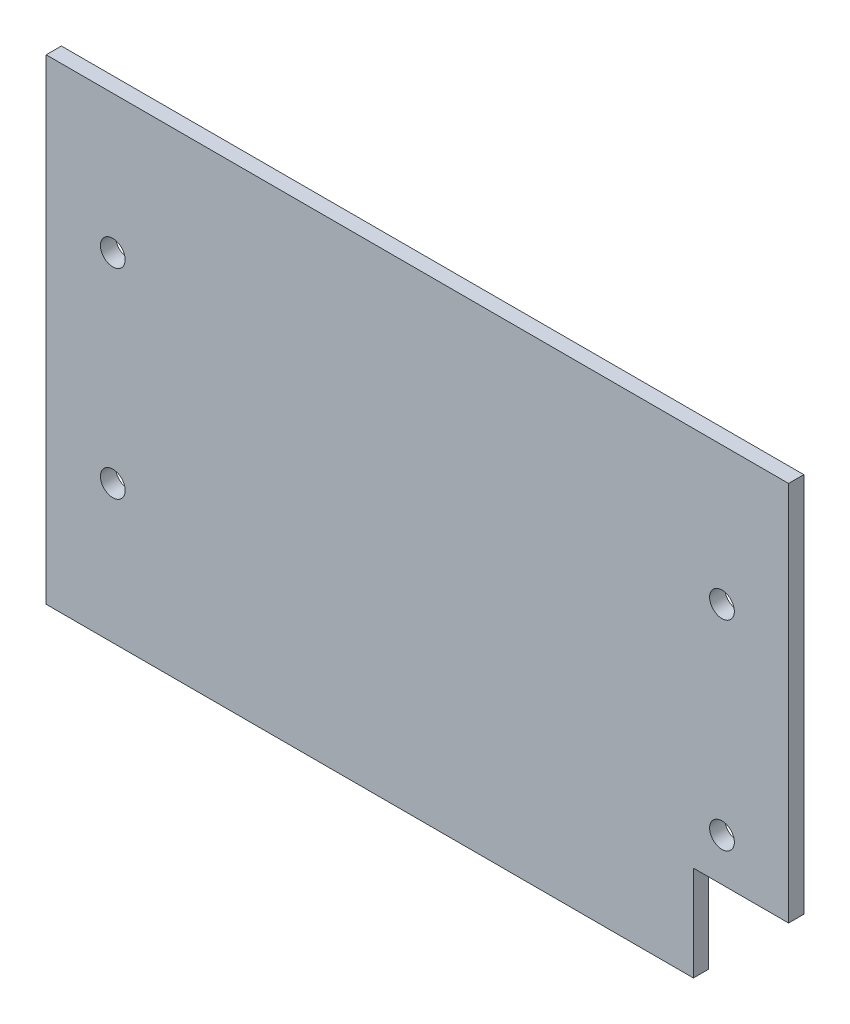
from build123d import *

# Parameters (mm, degrees)
SKETCH_1_W          = 390
SKETCH_1_H          = 250
EXTRUDE_1_DEPTH     = 8
CUT_EXTRUDE_1_DEPTH = 8
SKETCH_3_W          = 50
SKETCH_3_H          = 50
CUT_EXTRUDE_2_DEPTH = 60


with BuildPart() as part:
    # 草图1 → 凸台-拉伸1 (new body)
    with BuildSketch(Plane.XY):
        with Locations((195, 125)):
            Rectangle(SKETCH_1_W, SKETCH_1_H)
    extrude(amount=EXTRUDE_1_DEPTH)

    # 草图2 → 切除-拉伸1 (cut)
    with BuildSketch(Plane.XY.offset(8)):
        with BuildLine():
            ThreePointArc((41.5, 177.5), (30.403805922, 182.096194078), (35, 171))
            Line((35, 171), (35, 177.5))
            Line((35, 177.5), (41.5, 177.5))
        make_face()
        with BuildLine():
            Line((35, 177.5), (35, 171))
            ThreePointArc((35, 171), (39.596194078, 172.903805922), (41.5, 177.5))
            Line((41.5, 177.5), (35, 177.5))
        make_face()
        with BuildLine():
            Line((35, 79), (35, 72.5))
            Line((35, 72.5), (41.5, 72.5))
            ThreePointArc((41.5, 72.5), (39.596194078, 77.096194078), (35, 79))
        make_face()
        with BuildLine():
            Line((41.5, 72.5), (35, 72.5))
            Line((35, 72.5), (35, 79))
            ThreePointArc((35, 79), (30.403805922, 67.903805922), (41.5, 72.5))
        make_face()
        with BuildLine():
            ThreePointArc((355, 79), (350.403805922, 77.096194078), (348.5, 72.5))
            Line((348.5, 72.5), (355, 72.5))
            Line((355, 72.5), (355, 79))
        make_face()
        with BuildLine():
            Line((355, 72.5), (348.5, 72.5))
            ThreePointArc((348.5, 72.5), (355, 66), (361.5, 72.5))
            ThreePointArc((361.5, 72.5), (359.596194078, 77.096194078), (355, 79))
            Line((355, 79), (355, 72.5))
        make_face()
        with BuildLine():
            ThreePointArc((348.5, 177.5), (350.403805922, 172.903805922), (355, 171))
            Line((355, 171), (355, 177.5))
            Line((355, 177.5), (348.5, 177.5))
        make_face()
        with BuildLine():
            Line((355, 177.5), (355, 171))
            ThreePointArc((355, 171), (359.596194078, 172.903805922), (361.5, 177.5))
            ThreePointArc((361.5, 177.5), (355, 184), (348.5, 177.5))
            Line((348.5, 177.5), (355, 177.5))
        make_face()
    extrude(amount=-CUT_EXTRUDE_1_DEPTH, mode=Mode.SUBTRACT)

    # 草图3 → 切除-拉伸2 (cut)
    with BuildSketch(Plane.XY.offset(8)):
        with Locations((365, 25)):
            Rectangle(SKETCH_3_W, SKETCH_3_H)
    extrude(amount=-CUT_EXTRUDE_2_DEPTH, mode=Mode.SUBTRACT)


solid = part.part
